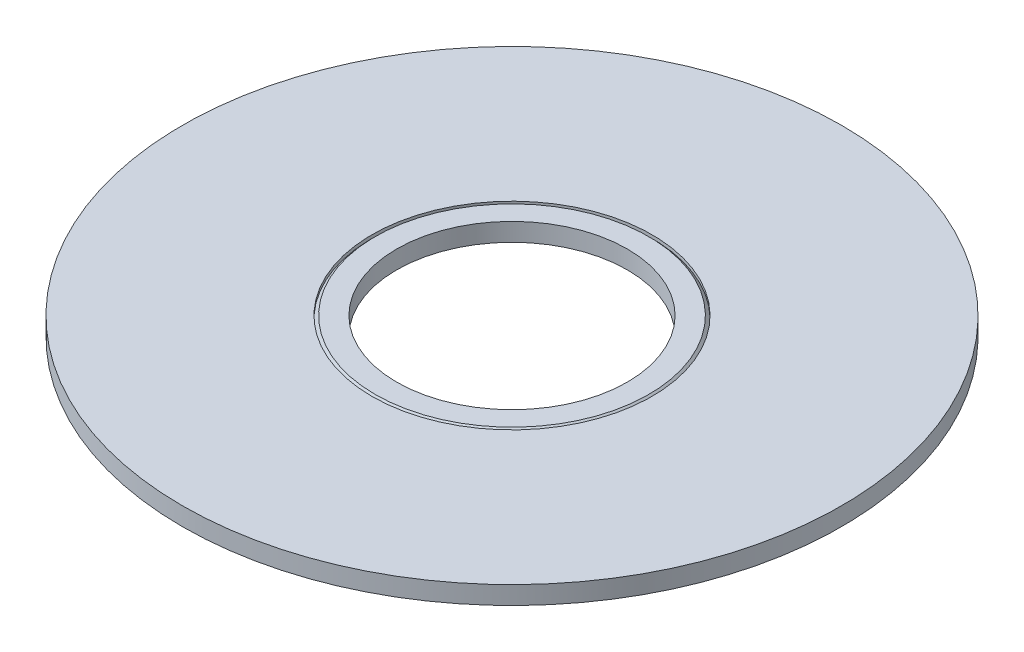
SolidWorks part; units mm, degrees
ref_plane "Front Plane" through (0, 0, 0) normal (0, 0, 1) x (1, 0, 0)
ref_plane "Top Plane" through (0, 0, 0) normal (0, 1, 0) x (1, 0, 0)
ref_plane "Right Plane" through (0, 0, 0) normal (1, 0, 0) x (0, 0, -1)
sketch "Sketch1" plane through (0, 0, 0) normal (0, 1, 0) x (1, 0, 0)
  circle A0 centre (0, 0) radius 42.5
  circle A1 centre (0, 0) radius 35
  dimension "D1" = 70
  dimension "D2" = 85
extrude "Boss-Extrude1" add sketch "Sketch1" along normal blind 5.5
chamfer "Chamfer1" distance 1 angle 45 2 edges at (0, 0, 42.5) (0, 5.5, 42.5)
sketch "Sketch2" plane through (0, 5.5, 0) normal (0, 1, 0) x (1, 0, 0)
  circle A0 centre (0, 0) radius 42.5
  circle A1 centre (0, 0) radius 100
  dimension "D1" = 200
extrude "Boss-Extrude2" add sketch "Sketch2" against normal blind 5.5
